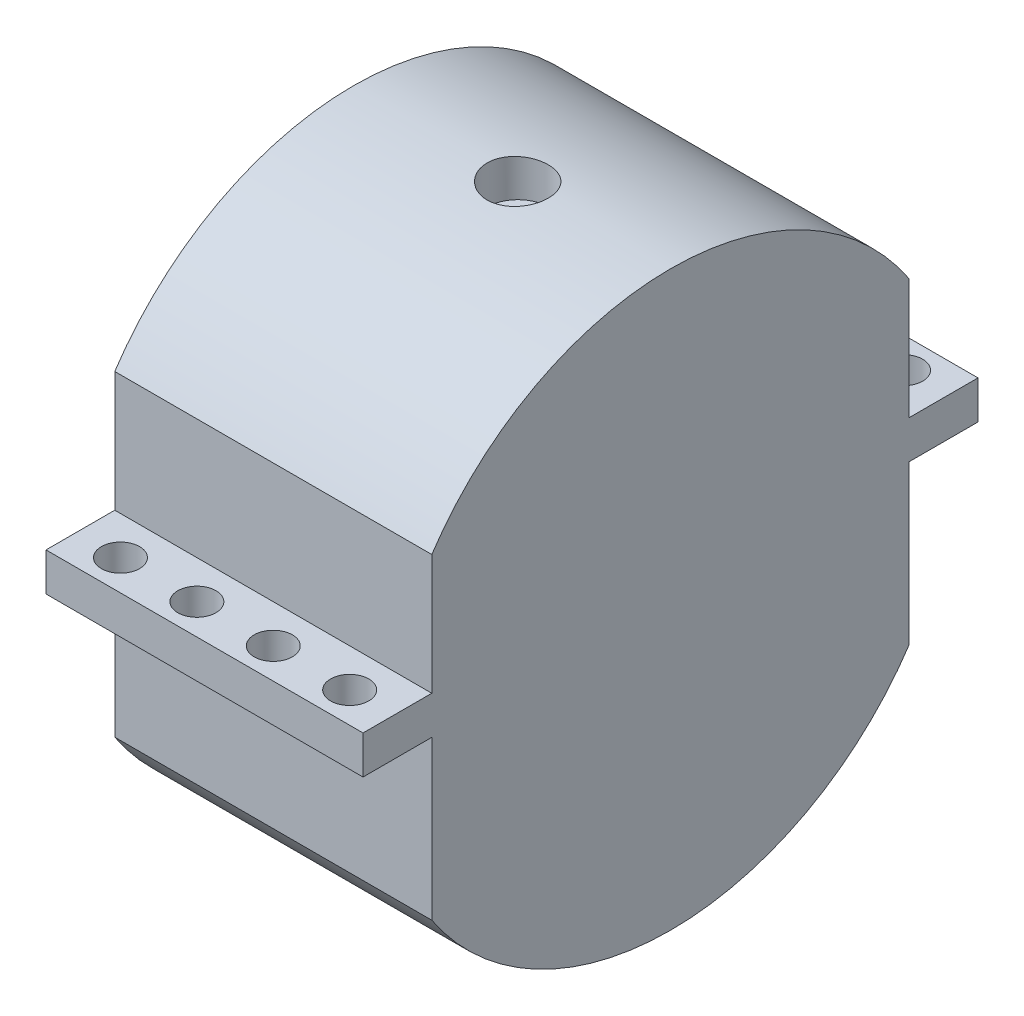
SolidWorks part; units mm, degrees
ref_plane "前视基准面" through (0, 0, 0) normal (0, 0, 1) x (1, 0, 0)
ref_plane "上视基准面" through (0, 0, 0) normal (0, 1, 0) x (1, 0, 0)
ref_plane "右视基准面" through (0, 0, 0) normal (1, 0, 0) x (0, 0, -1)
sketch "草图1" plane through (0, 0, 0) normal (0, 0, 1) x (1, 0, 0)
  line L0 (-130.3704, 0) -> (221.6296, 0) construction
  line L1 (30.7778, 50) -> (30.7778, 75)
  line L2 (30.7778, 75) -> (113.7778, 75)
  line L3 (113.7778, 75) -> (113.7778, 0)
  line L4 (113.7778, 0) -> (93.7778, 0)
  line L5 (93.7778, 0) -> (93.7778, 30)
  line L6 (93.7778, 30) -> (95.7778, 32)
  line L7 (95.7778, 32) -> (95.7778, 40)
  line L8 (95.7778, 40) -> (43.7778, 40)
  line L9 (43.7778, 40) -> (43.7778, 50)
  line L10 (43.7778, 50) -> (30.7778, 50)
  dimension "D1" = 8
  dimension "D2" = 30
  dimension "D3" = 20
  dimension "D4" = 18
  dimension "D5" = 83
  dimension "D6" = 10
  dimension "D7" = 13
  dimension "D8" = 25
  dimension "D9" = 135
revolve "旋转1" add sketch "草图1" angle 360 about L0
sketch "草图6" plane through (113.7778, 0, 0) normal (1, 0, 0) x (0, 0, -1)
  line L0 (0, 91.3596) -> (0, -84.1426) construction
  line L1 (62.5, 41.4578) -> (62.5, -41.4578)
  line L2 (-62.5, 41.4578) -> (-62.5, -41.4578)
  arc A0 (-62.5, 41.4578) -> (-62.5, -41.4578) centre (0, 0) ccw
  arc A1 (62.5, -41.4578) -> (62.5, 41.4578) centre (0, 0) ccw
  dimension "D1" = 62.5
extrude "切除-拉伸1" cut sketch "草图6" against normal up to next
sketch "草图9" plane through (113.7778, 0, 0) normal (1, 0, 0) x (0, 0, -1)
  line L0 (-62.5, 0) -> (-80.5, 0)
  line L1 (-62.5, -41.4578) -> (-62.5, 41.4578) construction
  line L2 (-80.5, 0) -> (-80.5, 10)
  line L3 (-80.5, 10) -> (-62.5, 10)
  line L4 (-62.5, 10) -> (-62.5, 0)
  line L5 (0, 64.608) -> (0, -84.6415) construction
  line L6 (62.5, 10) -> (62.5, 0)
  line L7 (62.5, 0) -> (80.5, 0)
  line L8 (80.5, 0) -> (80.5, 10)
  line L9 (80.5, 10) -> (62.5, 10)
  dimension "D1" = 18
  dimension "D2" = 10
extrude "凸台-拉伸1" add sketch "草图9" against normal up to surface (83 mm away) up to face at (30.7778, 0, 50)
sketch "草图10" plane through (0, 10, 0) normal (0, 1, 0) x (1, 0, 0)
  line L0 (0, 0) -> (182.6618, 0) construction
  line L2 (30.7778, 62.5) -> (30.7778, 80.5) construction
  circle A0 centre (42.2778, 72.5) radius 5
  circle A1 centre (62.2778, 72.5) radius 5
  circle A2 centre (82.2778, 72.5) radius 5
  circle A3 centre (102.2778, 72.5) radius 5
  circle A4 centre (102.2778, -72.5) radius 5
  circle A5 centre (82.2778, -72.5) radius 5
  circle A6 centre (62.2778, -72.5) radius 5
  circle A7 centre (42.2778, -72.5) radius 5
  dimension "D1" = 10
  dimension "D2" = 72.5
  dimension "D3" = 72.5
  dimension "D4" = 72.5
  dimension "D5" = 72.5
  dimension "D6" = 20
  dimension "D7" = 20
  dimension "D8" = 20
  dimension "D9" = 11.5
extrude "切除-拉伸4" cut sketch "草图10" against normal up to next
ref_plane "基准面1" through (0, 75, 0) normal (0, 1, 0) x (1, 0, 0)
sketch "草图11" plane through (0, 75, 0) normal (0, 1, 0) x (1, 0, 0)
  line L0 (113.7778, -62.5) -> (113.7778, 62.5) construction
  circle A0 centre (73.7778, 0) radius 5
  dimension "D1" = 40
  dimension "D2" = 10
extrude "切除-拉伸5" cut sketch "草图11" against normal up to next
sketch "草图12" plane through (0, 75, 0) normal (0, 1, 0) x (1, 0, 0)
  circle A0 centre (73.7778, 0) radius 8
  dimension "D1" = 16
extrude "切除-拉伸6" cut sketch "草图12" against normal blind 10
